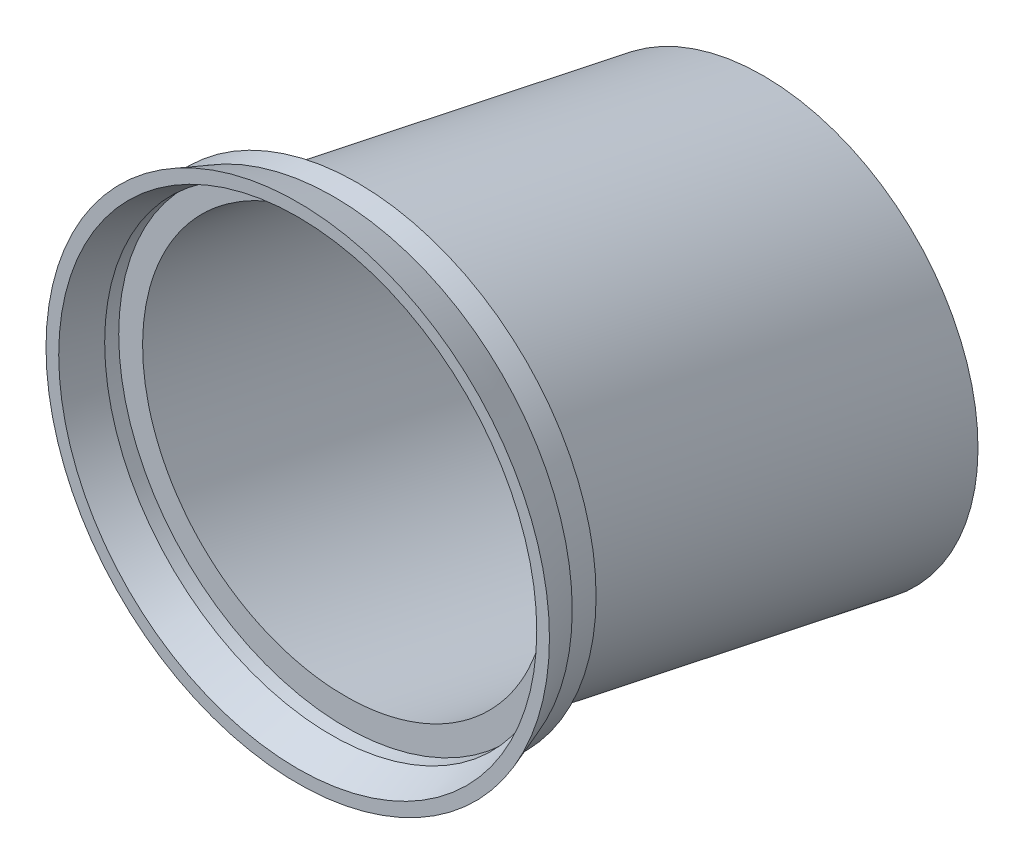
SolidWorks part; units mm, degrees
ref_plane "前视基准面" through (0, 0, 0) normal (0, 0, 1) x (1, 0, 0)
ref_plane "上视基准面" through (0, 0, 0) normal (0, 1, 0) x (1, 0, 0)
ref_plane "右视基准面" through (0, 0, 0) normal (1, 0, 0) x (0, 0, -1)
sketch "草图1" plane through (0, 0, 0) normal (0, 0, 1) x (1, 0, 0)
  circle A0 centre (0, 0) radius 20
  dimension "D1" = 40
extrude "凸台-拉伸1" add sketch "草图1" along normal blind 3 draft 20 and the other way blind 2
sketch "草图2" plane through (0, 0, -2) normal (0, 0, -1) x (-1, 0, 0)
  circle A0 centre (0, 0) radius 18
  dimension "D1" = 36
sketch "草图3" plane through (0, 0, 0) normal (1, 0, 0) x (0, 0, -1)
  line L0 (-19.9298, 0) -> (59.9727, 0) construction
  line L1 (2, 0) -> (46.0166, -9.356)
  line L2 (2, -18) -> (2, 18) construction
  dimension "D1" = 12
  dimension "D2" = 45
sweep "扫描1" add profiles "草图2" path "草图3"
sketch "草图5" plane through (0, 0, -2) normal (0, 0, -1) x (-1, 0, 0)
  circle A0 centre (0, 0) radius 37.5413
extrude "切除-拉伸1" cut sketch "草图5" along normal blind 53 from offset 34
shell "抽壳1" thickness 1
